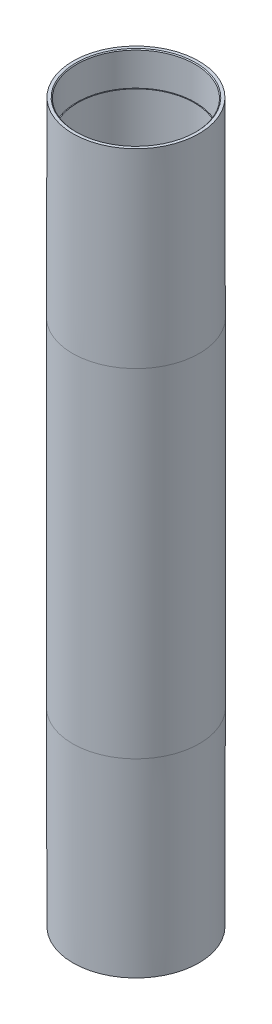
SolidWorks part; units mm, degrees
material "1023 碳钢板 (SS)"
ref_plane "前视基准面" through (0, 0, 0) normal (0, 0, 1) x (1, 0, 0)
ref_plane "上视基准面" through (0, 0, 0) normal (0, 1, 0) x (1, 0, 0)
ref_plane "右视基准面" through (0, 0, 0) normal (1, 0, 0) x (0, 0, -1)
sketch "草图1" plane through (0, 0, 0) normal (0, 0, 1) x (1, 0, 0)
  line L0 (0, 0) -> (-0.5, 225)
  line L1 (-0.5, 225) -> (-0.5, 625)
  line L2 (-0.5, 625) -> (0, 850)
  line L3 (0, 850) -> (74.5, 850)
  line L4 (0, 0) -> (74.5, 0)
  line L5 (74.5, 850) -> (74.5, 737.8515) construction
  line L6 (74.5, 0) -> (74.5, 850)
  dimension "D1" = 400
  dimension "D2" = 225
  dimension "D3" = 225
  dimension "D4" = 74.5
  dimension "D5" = 75
revolve "旋转1" add sketch "草图1" angle 360 about L5
sketch "草图2" plane through (0, 850, 0) normal (0, 1, 0) x (1, 0, 0)
  circle A0 centre (74.5, 0) radius 70
  dimension "D1" = 140
extrude "切除-拉伸1" cut sketch "草图2" against normal blind 40
sketch "草图3" plane through (0, 0, 0) normal (0, -1, 0) x (1, 0, 0)
  circle A0 centre (74.5, 0) radius 70
  dimension "D1" = 140
extrude "切除-拉伸2" cut sketch "草图3" against normal blind 40
sketch "草图4" plane through (0, 40, 0) normal (0, -1, 0) x (1, 0, 0)
  circle A0 centre (74.5, 0) radius 69
  dimension "D1" = 138
extrude "切除-拉伸3" cut sketch "草图4" against normal blind 843
chamfer "倒角1" distance 1 angle 45 2 edges at (74.5, 850, 70) (74.5, 0, -70)
